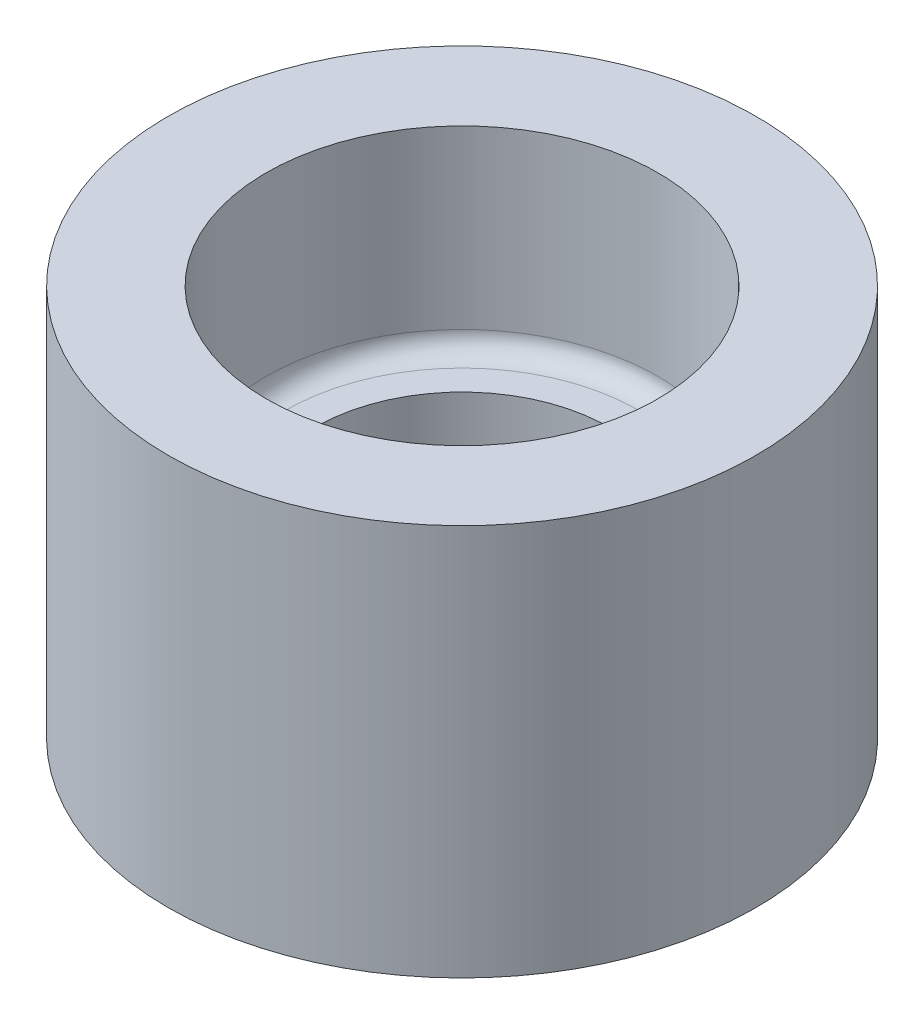
from build123d import *


with BuildPart() as part:
    # 草图1 → 旋转1 (revolve)
    with BuildSketch(Plane.XY, mode=Mode.PRIVATE) as revolve_1_sk:
        with BuildLine():
            Line((15, -20), (15, 0))
            Line((15, 0), (18, 0))
            ThreePointArc((18, 0), (19.414213562, 0.585786438), (20, 2))
            Line((20, 2), (20, 20))
            Line((20, 20), (30, 20))
            Line((30, 20), (30, -20))
            Line((30, -20), (15, -20))
        make_face()
    revolve(revolve_1_sk.sketch.rotate(Axis((0, 45.568181818, 0), (0, -1, 0)), 90), axis=Axis((0, 45.568181818, 0), (0, -1, 0)))


solid = part.part
